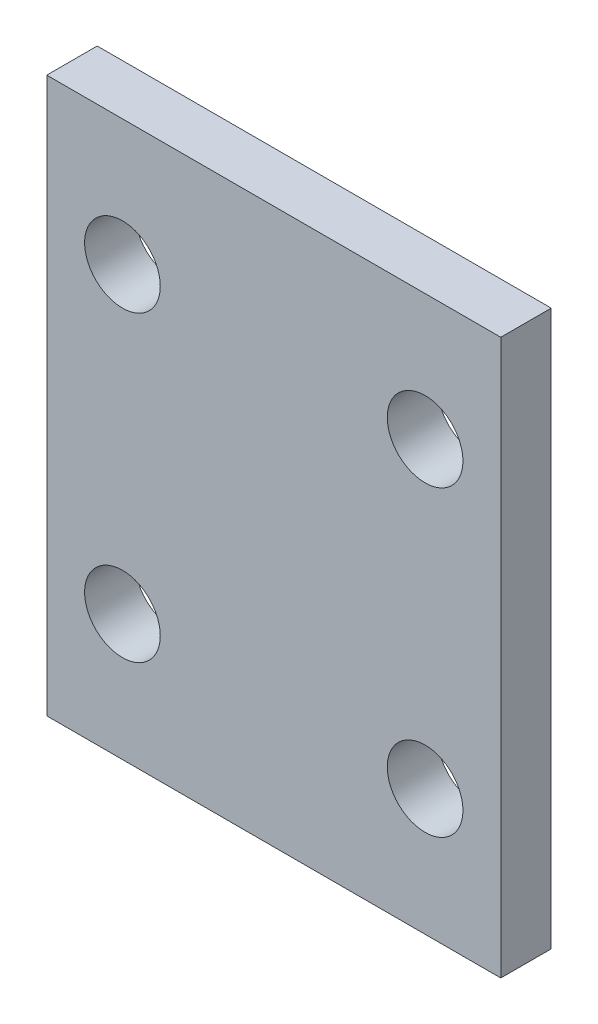
SolidWorks part; units mm, degrees
ref_plane "前视基准面" through (0, 0, 0) normal (0, 0, 1) x (1, 0, 0)
ref_plane "上视基准面" through (0, 0, 0) normal (0, 1, 0) x (1, 0, 0)
ref_plane "右视基准面" through (0, 0, 0) normal (1, 0, 0) x (0, 0, -1)
sketch "草图1" plane through (0, 0, 0) normal (0, 0, 1) x (1, 0, 0)
  line L0 (0, 0) -> (0, 120)
  line L1 (0, 120) -> (100, 120)
  line L2 (100, 120) -> (100, 0)
  line L3 (100, 0) -> (0, 0)
extrude "凸台-拉伸1" add sketch "草图1" along normal blind 10
sketch "草图2" plane through (0, 0, 10) normal (0, 0, 1) x (1, 0, 0)
  line L0 (20, 60) -> (20, 90)
  line L1 (20, 90) -> (80, 90)
  line L6 (80, 90) -> (80, 30)
  line L7 (80, 30) -> (20, 30)
  line L8 (20, 30) -> (20, 60)
  circle A0 centre (20, 90) radius 7.5
  circle A1 centre (80, 90) radius 7.5
  circle A2 centre (80, 30) radius 7.5
  circle A3 centre (20, 30) radius 7.5
extrude "切除-拉伸1" cut sketch "草图2" against normal blind 10 contours L6 A1 L1 | L1 A1 L6 | L1 A0 L0 | L0 A0 L1 | L8 A3 L7 | L7 A3 L8 | L6 A2 L7 | L7 A2 L6
cosmetic thread "装饰螺纹线1" parameters "D2"=17
cosmetic thread "装饰螺纹线2" parameters "D2"=17
cosmetic thread "装饰螺纹线3" parameters "D2"=17
cosmetic thread "装饰螺纹线4" parameters "D2"=17
sketch "草图3" plane through (0, 0, 10) normal (0, 0, 1) x (1, 0, 0)
  line L5 (95, 60) -> (95, 5)
  line L6 (95, 60) -> (95, 115)
  line L7 (95, 115) -> (5, 115)
  line L8 (5, 115) -> (5, 5)
  line L9 (5, 5) -> (95, 5)
  line L15 (0, 0) -> (100, 0)
  line L16 (100, 0) -> (100, 120)
  line L17 (100, 120) -> (0, 120)
  line L18 (0, 120) -> (0, 0)
  line L19 (0, 0) -> (100, 0)
  line L20 (100, 0) -> (100, 120)
  line L21 (100, 120) -> (0, 120)
  line L22 (0, 120) -> (0, 0)
  dimension "D1" = 0
extrude "切除-拉伸2" cut sketch "草图3" against normal blind 10
